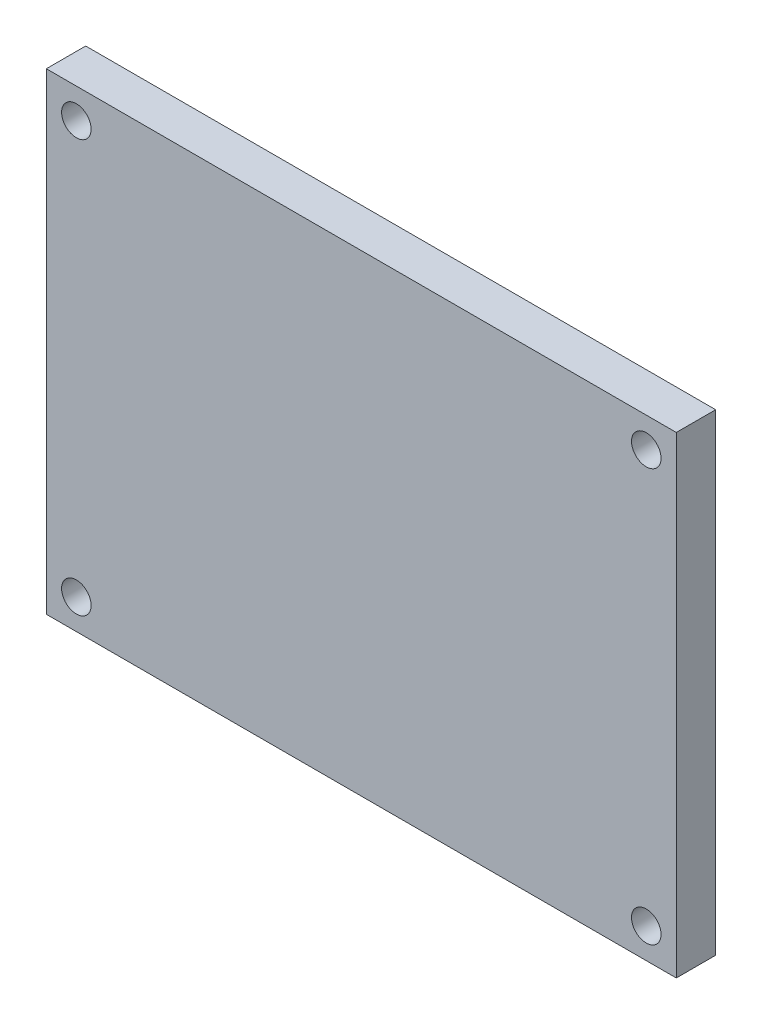
SolidWorks part; units mm, degrees
ref_plane "Front Plane" through (0, 0, 0) normal (0, 0, 1) x (1, 0, 0)
ref_plane "Top Plane" through (0, 0, 0) normal (0, 1, 0) x (1, 0, 0)
ref_plane "Right Plane" through (0, 0, 0) normal (1, 0, 0) x (0, 0, -1)
other "Configuration Table"
sketch "Sketch1" plane through (0, 0, 0) normal (0, 0, 1) x (1, 0, 0)
  line L1 (-32, -24) -> (32, -24)
  line L2 (-32, -24) -> (-32, 24)
  line L3 (-32, 24) -> (32, 24)
  line L4 (32, -24) -> (32, 24)
  line L5 (0, 24) -> (0, -24) construction
  line L6 (-32, 0) -> (32, 0) construction
  point P0 (0, 0)
  dimension "D1" = 64
  dimension "D2" = 48
extrude "Boss-Extrude1" add sketch "Sketch1" along normal blind 4
sketch "Sketch2" plane through (0, 0, 4) normal (0, 0, 1) x (1, 0, 0)
  line L1 (28.95, 20.95) -> (-28.95, 20.95) construction
  line L2 (28.95, 20.95) -> (28.95, -20.95) construction
  line L3 (28.95, -20.95) -> (-28.95, -20.95) construction
  line L4 (-28.95, 20.95) -> (-28.95, -20.95) construction
  line L5 (0, -20.95) -> (0, 20.95) construction
  line L6 (28.95, 0) -> (-28.95, 0) construction
  circle A0 centre (28.95, -20.95) radius 1.5
  circle A1 centre (-28.95, -20.95) radius 1.5
  circle A2 centre (28.95, 20.95) radius 1.5
  circle A3 centre (-28.95, 20.95) radius 1.5
  point P0 (0, 0)
  dimension "D3" = 3
  dimension "D1" = 57.9
  dimension "D2" = 41.9
extrude "Cut-Extrude1" cut sketch "Sketch2" against normal through all both
